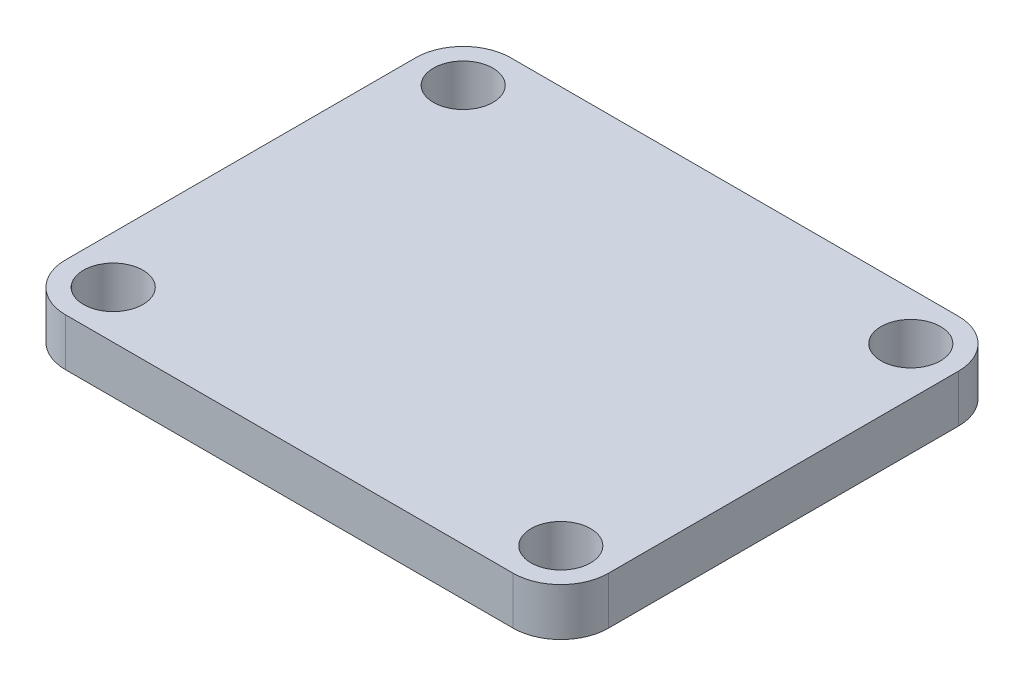
SolidWorks part; units mm, degrees
ref_plane "Front Plane" through (0, 0, 0) normal (0, 0, 1) x (1, 0, 0)
ref_plane "Top Plane" through (0, 0, 0) normal (0, 1, 0) x (1, 0, 0)
ref_plane "Right Plane" through (0, 0, 0) normal (1, 0, 0) x (0, 0, -1)
sketch "Sketch1" plane through (0, 0, 0) normal (0, 0, 1) x (1, 0, 0)
  line L0 (51.1656, 84.9757) -> (42.1853, 93.9559)
  line L1 (42.1853, 93.9559) -> (42.1853, 113.634)
extrude "Extrude-Thin1" add sketch "Sketch1" against normal blind 12.7 thin thin type one direction reverse wall 2
sketch "Sketch3" plane through (0, 113.634, 0) normal (0, 1, 0) x (1, 0, 0)
  line L0 (51.1656, 6.35) -> (40.1853, 6.35) construction
  line L5 (51.1656, 12.7) -> (51.1656, 0) construction
  line L7 (40.1853, 12.7) -> (40.1853, 0) construction
  line L8 (40.1853, 6.35) -> (45.6754, 6.35) construction
  line L9 (45.6754, 6.35) -> (45.6754, 13.9713) construction
  line L11 (57.0754, 15.7) -> (34.2754, 15.7)
  line L12 (57.0754, 15.7) -> (57.0754, -3)
  line L13 (57.0754, -3) -> (34.2754, -3)
  line L14 (34.2754, 15.7) -> (34.2754, -3)
  dimension "D1" = 5.9099
  dimension "D2" = 22.8
  dimension "D3" = 18.7
extrude "Boss-Extrude2" add sketch "Sketch3" along normal blind 2 separate body
fillet "Fillet1" radius 2 4 edges at (57.0754, 114.634, 3) (34.2754, 114.634, 3) (34.2754, 114.634, -15.7) (57.0754, 114.634, -15.7)
sketch "Sketch4" plane through (0, 115.634, 0) normal (0, 1, 0) x (1, 0, 0)
  circle A0 centre (55.0754, 13.7) radius 1.25
  circle A1 centre (55.0754, -1) radius 1.25
  circle A2 centre (36.2754, -1) radius 1.25
  circle A3 centre (36.2754, 13.7) radius 1.25
  dimension "D1" = 2.5
extrude "Cut-Extrude1" cut sketch "Sketch4" against normal blind 2
sketch "Sketch5" plane through (68.0706, 68.0706, 0) normal (0.7071, 0.7071, 0) x (0, 0, -1)
  circle A0 centre (6.35, 30.2574) radius 2.75
  dimension "D1" = 5.5
extrude "Cut-Extrude2" cut sketch "Sketch5" against normal through all both and the other way through all
sketch "Sketch6" plane through (66.6564, 66.6564, 0) normal (-0.7071, -0.7071, 0) x (0, 0, 1)
  circle A0 centre (-10.65, 34.5574) radius 1.25
  circle A1 centre (-2.05, 34.5574) radius 1.25
  circle A2 centre (-2.05, 25.9574) radius 1.25
  circle A3 centre (-10.65, 25.9574) radius 1.25
  dimension "D1" = 2.5
extrude "Cut-Extrude3" cut sketch "Sketch6" against normal blind 10
sketch "Sketch7" plane through (0, 0, 3) normal (0, 0, 1) x (1, 0, 0)
  line L1 (55.0754, 113.634) -> (33.8654, 113.634)
  line L2 (55.0754, 113.634) -> (55.0754, 81.1365)
  line L3 (55.0754, 81.1365) -> (33.8654, 81.1365)
  line L4 (33.8654, 113.634) -> (33.8654, 81.1365)
extrude "Cut-Extrude4" cut sketch "Sketch7" against normal through all both and the other way through all
